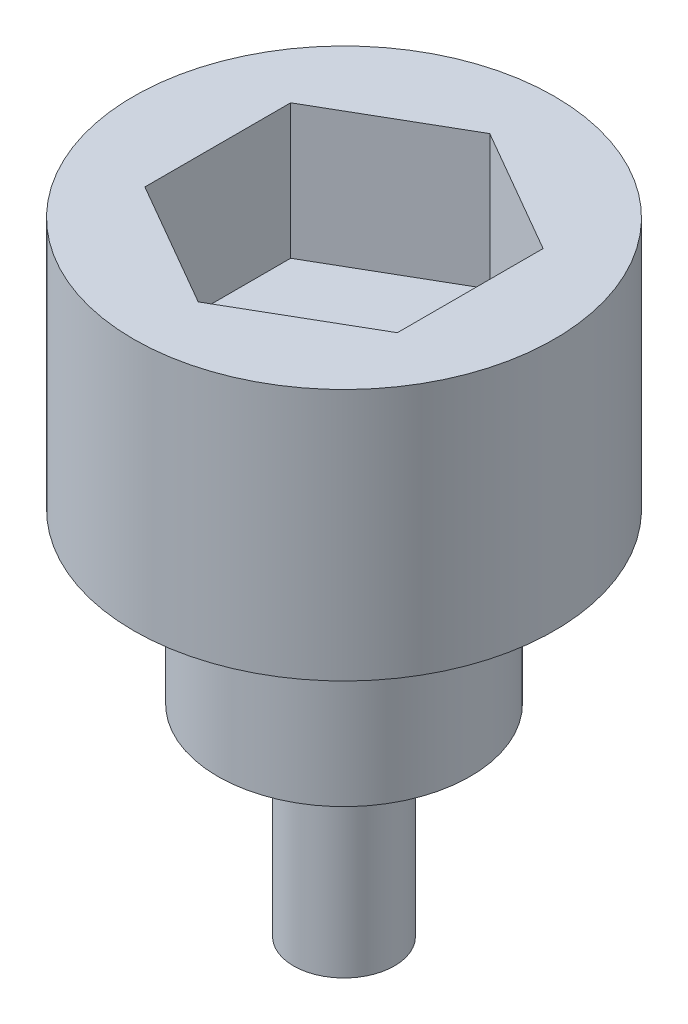
from build123d import *

# Parameters (mm, degrees)
SKETCH1_R           = 3
BOSS_EXTRUDE1_DEPTH = 12
SKETCH2_R           = 7.5
BOSS_EXTRUDE2_DEPTH = 10
SKETCH3_R           = 12.5
BOSS_EXTRUDE3_DEPTH = 15
CUT_EXTRUDE1_DEPTH  = 8


with BuildPart() as part:
    # Sketch1 → Boss-Extrude1 (new body)
    with BuildSketch(Plane(origin=(0, 0, 0), x_dir=(1, 0, 0), z_dir=(0, 1, 0))):
        with Locations(Location((0, 0, 0), (0, 0, 270))):
            Circle(SKETCH1_R)
    extrude(amount=BOSS_EXTRUDE1_DEPTH)

    # Sketch2 → Boss-Extrude2 (add)
    with BuildSketch(Plane(origin=(0, 12, 0), x_dir=(1, 0, 0), z_dir=(0, 1, 0))):
        with Locations(Location((0, 0, 0), (0, 0, 270))):
            Circle(SKETCH2_R)
    extrude(amount=BOSS_EXTRUDE2_DEPTH)

    # Sketch3 → Boss-Extrude3 (add)
    with BuildSketch(Plane(origin=(0, 22, 0), x_dir=(1, 0, 0), z_dir=(0, 1, 0))):
        with Locations(Location((0, 0, 0), (0, 0, 270))):
            Circle(SKETCH3_R)
    extrude(amount=BOSS_EXTRUDE3_DEPTH)

    # Sketch4 → Cut-Extrude1 (cut)
    with BuildSketch(Plane(origin=(0, 37, 0), x_dir=(1, 0, 0), z_dir=(0, 1, 0))):
        Polygon((0, 8.660254038), (-7.5, 4.330127019), (-7.5, -4.330127019), (0, -8.660254038), (7.5, -4.330127019), (7.5, 4.330127019), align=None)
    extrude(amount=-CUT_EXTRUDE1_DEPTH, mode=Mode.SUBTRACT)


solid = part.part
